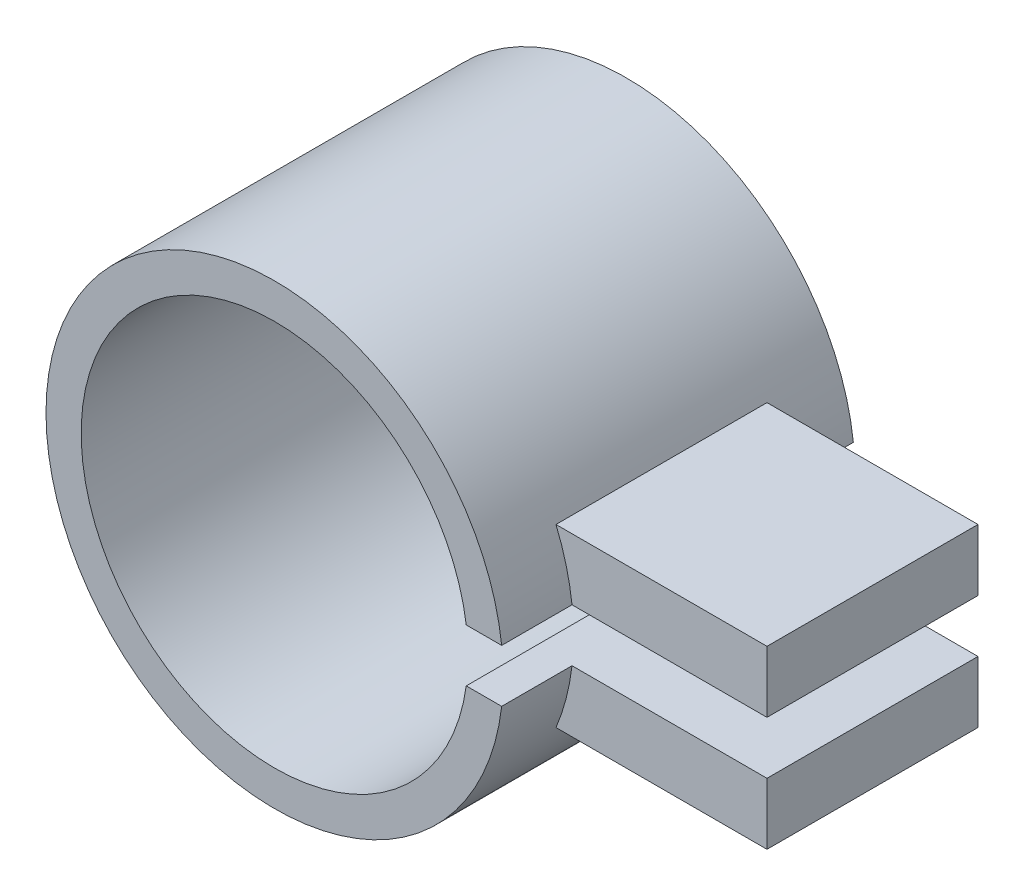
from build123d import *

# Parameters (mm, degrees)
SKETCH1_R           = 6.5
SKETCH1_R_2         = 5.5
EXTRUDE_THIN1_DEPTH = 5
SKETCH2_W           = 6
SKETCH2_H           = 5
BOSS_EXTRUDE1_DEPTH = 3
SKETCH4_W           = 14.223079102
SKETCH4_H           = 1.5
CUT_EXTRUDE1_DEPTH  = 17.918924316


with BuildPart() as part:
    # Sketch1 → Extrude-Thin1 (new, symmetric)
    with BuildSketch(Plane.XY):
        Circle(SKETCH1_R)
        Circle(SKETCH1_R_2, mode=Mode.SUBTRACT)
    extrude(amount=EXTRUDE_THIN1_DEPTH, both=True)

    # Sketch2 → Boss-Extrude1 (add, symmetric)
    with BuildSketch(Plane.XY):
        with Locations((9, 0)):
            Rectangle(SKETCH2_W, SKETCH2_H)
    extrude(amount=BOSS_EXTRUDE1_DEPTH, both=True)

    # Sketch4 → Cut-Extrude1 (cut, through all)
    with BuildSketch(Plane.XY.offset(5)):
        with Locations((7.111539551, 0)):
            Rectangle(SKETCH4_W, SKETCH4_H)
    extrude(amount=-CUT_EXTRUDE1_DEPTH, mode=Mode.SUBTRACT)


solid = part.part
